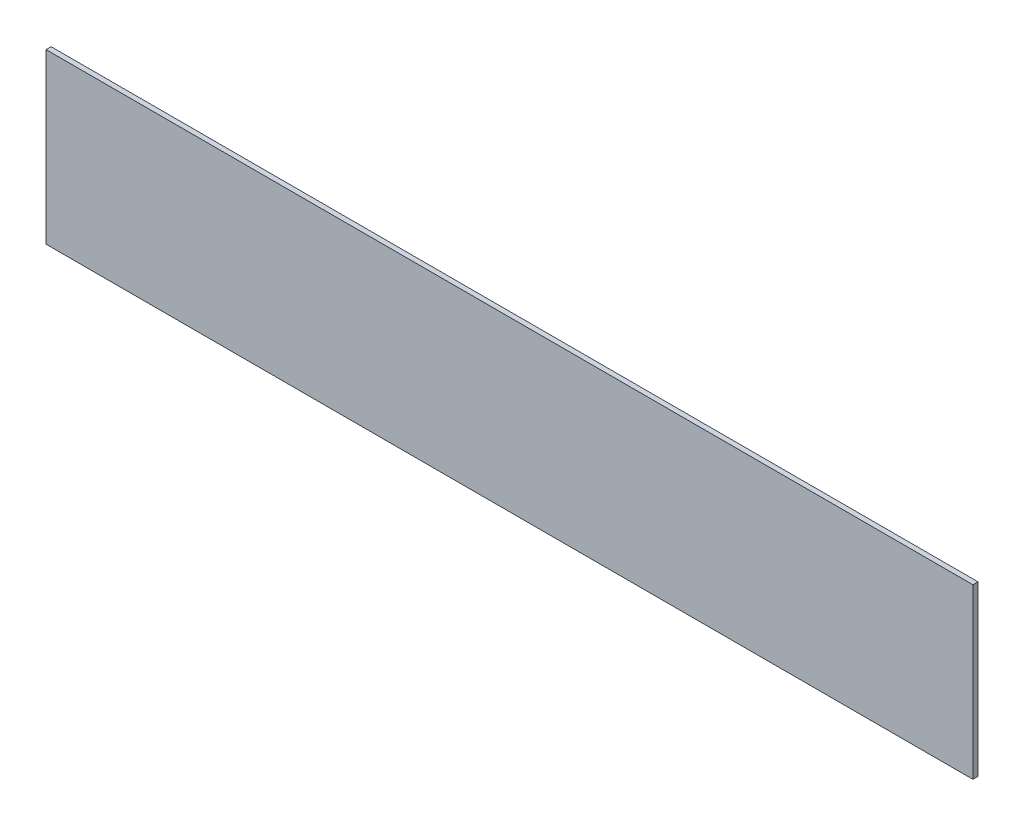
from build123d import *

# Parameters (mm, degrees)
SKETCH_1_W      = 550
SKETCH_1_H      = 100
EXTRUDE_1_DEPTH = 3


with BuildPart() as part:
    # 草图1 → 凸台-拉伸1 (new body)
    with BuildSketch(Plane.XY):
        Rectangle(SKETCH_1_W, SKETCH_1_H)
    extrude(amount=EXTRUDE_1_DEPTH)


solid = part.part
